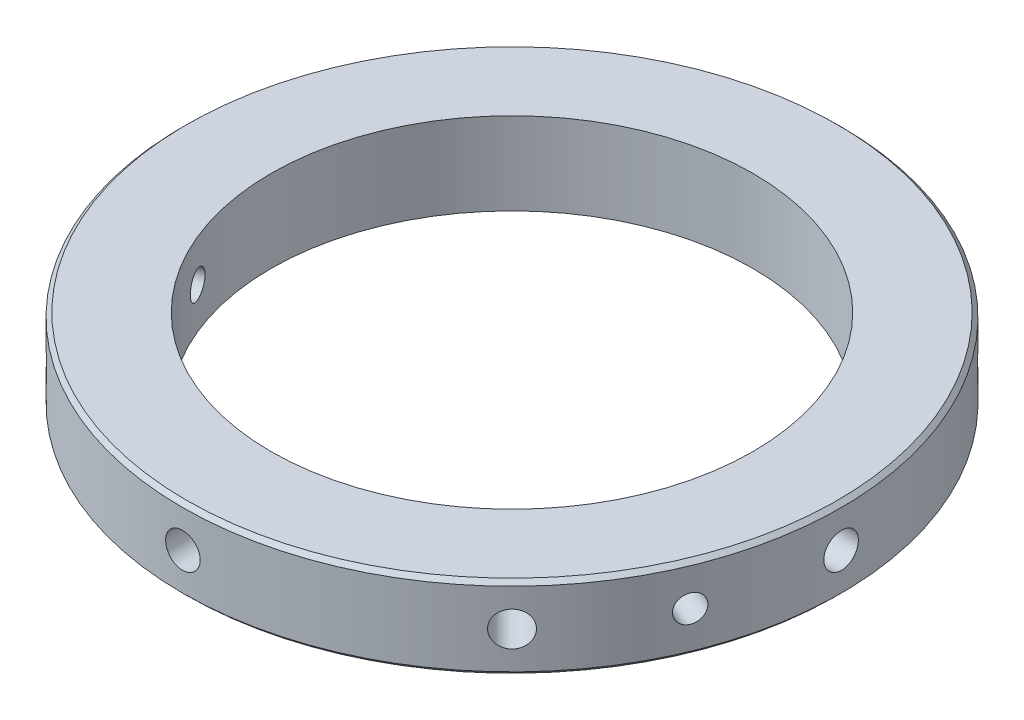
SolidWorks part; units mm, degrees
ref_plane "Front Plane" through (0, 0, 0) normal (0, 0, 1) x (1, 0, 0)
ref_plane "Top Plane" through (0, 0, 0) normal (0, 1, 0) x (1, 0, 0)
ref_plane "Right Plane" through (0, 0, 0) normal (1, 0, 0) x (0, 0, -1)
sketch "Sketch1" plane through (0, 0, 0) normal (0, 1, 0) x (1, 0, 0)
  circle A0 centre (0, 0) radius 40
  circle A1 centre (0, 0) radius 29.25
  dimension "D1" = 80
  dimension "D2" = 58.5
extrude "Boss-Extrude1" add sketch "Sketch1" along normal mid plane 10
cosmetic thread "Cosmetic Thread1" parameters "D2"=60
ref_plane "Plane1" through (0, 0, 40) normal (0, 0, 1) x (1, 0, 0)
hole_wizard "Ø4.2 (4.2) Diameter Hole1" positions "Sketch3" profile "Sketch2" hole size "Ø4.2" standard "Gb"
sketch "Sketch3" plane through (0, 0, 40) normal (0, 0, 1) x (1, 0, 0)
  point P0 (0, 0)
sketch "Sketch2" plane through (0, 0, 40) normal (1, 0, 0) x (0, -1, 0)
  line L0 (0, 0) -> (0, 8.2618)
  line L1 (0, 8.2618) -> (2.1, 7)
  line L2 (2.1, 7) -> (2.1, 0)
  line L5 (2.1, 0) -> (0, 0)
  line L10 (0, 8.2618) -> (-2.1, 7) construction
  line L11 (0, -6.35) -> (0, 107.95) construction
  dimension "孔直径" = 4.2
  dimension "孔深度" = 7
  dimension "导头角度" = 118
pattern_circular "CirPattern1" count 8 over 360 about axis through (0, 5, 0) along (0, -1, 0) of "Ø4.2 (4.2) Diameter Hole1"
ref_plane "Plane2" through (36.9552, 0, 15.3073) normal (0.9239, 0, 0.3827) x (0.3827, 0, -0.9239)
hole_wizard "M4 Tapped Hole1" positions "Sketch5" profile "Sketch4" tap size "M4" standard "Gb"
sketch "Sketch5" plane through (36.9552, 0, 15.3073) normal (0.9239, 0, 0.3827) x (0.3827, 0, -0.9239)
  point P0 (0, 0)
sketch "Sketch4" plane through (36.9552, 0, 15.3073) normal (0, 1, 0) x (0.3827, 0, -0.9239)
  line L0 (0, 0) -> (0, 80)
  line L1 (0, 80) -> (1.65, 80)
  line L2 (1.65, 80) -> (1.65, 0)
  line L5 (1.65, 0) -> (0, 0)
  line L11 (0, -6.35) -> (0, 107.95) construction
  dimension "通孔螺纹孔钻头直径" = 3.3
  dimension "通孔螺纹孔钻头深度" = 80
cosmetic thread "Hole Cosmetic Thread1" parameters "D2"=4
pattern_circular "CirPattern2" count 2 every 135 about axis through (0, 5, 0) along (0, -1, 0) of "M4 Tapped Hole1"
chamfer "Chamfer1" distance 0.5 angle 45 2 edges at (0, -5, 40) (0, 5, 40)
